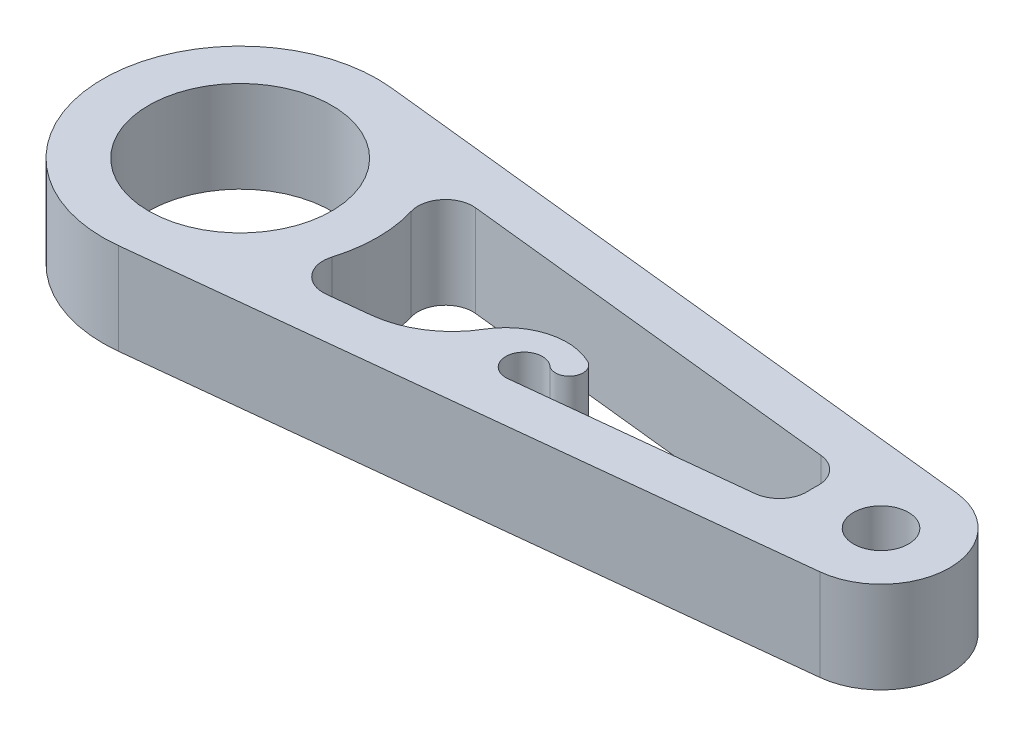
SolidWorks part; units mm, degrees
material "哈碳纤"
ref_plane "前视基准面" through (0, 0, 0) normal (0, 0, 1) x (1, 0, 0)
ref_plane "上视基准面" through (0, 0, 0) normal (0, 1, 0) x (1, 0, 0)
ref_plane "右视基准面" through (0, 0, 0) normal (1, 0, 0) x (0, 0, -1)
other "Configuration Table"
sketch "草图1" plane through (0, 0, 0) normal (0, 1, 0) x (1, 0, 0)
  line L0 (1.6071, 14.9137) -> (70.8036, 7.4568)
  line L1 (1.6071, -14.9137) -> (70.8036, -7.4568)
  line L2 (12.1874, 8.7445) -> (63.2375, 3.2432)
  line L3 (1.0714, 9.9424) -> (70.2679, 2.4856) construction
  line L4 (1.0714, -9.9424) -> (70.2679, -2.4856) construction
  line L5 (12.1874, -8.7445) -> (63.2375, -3.2432)
  circle A0 centre (0, 0) radius 10
  arc A1 (1.6071, 14.9137) -> (1.6071, -14.9137) centre (0, 0) ccw
  circle A2 centre (70, 0) radius 3
  arc A3 (70.8036, -7.4568) -> (70.8036, 7.4568) centre (70, 0) ccw
  arc A4 (12.1874, -8.7445) -> (12.1874, 8.7445) centre (0, 0) ccw
  arc A5 (63.2375, 3.2432) -> (63.2375, -3.2432) centre (70, 0) ccw
  dimension "D1" = 20
  dimension "D2" = 30
  dimension "D3" = 6
  dimension "D4" = 15
  dimension "D5" = 70
  dimension "D6" = 5
  dimension "D7" = 5
extrude "凸台-拉伸1" add sketch "草图1" along normal blind 10
fillet "圆角1" radius 3 4 edges at (63.2375, 5, 3.2432) (63.2375, 5, -3.2432) (12.1874, 5, 8.7445) (12.1874, 5, -8.7445)
sketch "草图2" plane through (0, 10, 0) normal (0, 1, 0) x (1, 0, 0)
  line L0 (-7.3229, 13.091) -> (-14.6458, 26.1821)
  line L2 (-14.6458, 26.1821) -> (-9.4094, 29.1112)
  line L3 (-9.4094, 29.1112) -> (1.6071, 14.9137)
  arc A0 (1.6071, 14.9137) -> (1.6071, -14.9137) centre (0, 0) ccw construction
  arc A1 (1.6071, 14.9137) -> (-7.3229, 13.091) centre (0, 0) ccw
  dimension "D2" = 30
  dimension "D3" = 6
extrude "凸台-拉伸2" [suppressed] add sketch "草图2" against normal blind 10
fillet "圆角2" [suppressed] radius 3
sketch "草图3" plane through (0, 10, 0) normal (0, 1, 0) x (1, 0, 0)
  line L0 (17.5591, -8.1657) -> (59.8401, -3.6093) construction
  line L1 (28.6131, -6.9745) -> (35.4729, -6.2352)
  arc A0 (36.559, -2.7272) -> (35.4729, -6.2352) centre (35.2586, -4.2467) ccw
  arc A1 (36.559, -2.7272) -> (38.1927, -0.2398) centre (37.5343, -1.5876) ccw
  arc A2 (38.1927, -0.2398) -> (28.6131, -6.9745) centre (35.2586, -6.2467) ccw
  circle A3 centre (70, 0) radius 3 construction
  point P1 (0, 0)
  point P3 (0, 0)
  point P13 (0, 0)
  point P14 (36.0991, -2.4319)
  point P15 (36.0955, -4.2741)
  dimension "D1" = 4
  dimension "D2" = 3
  dimension "D3" = 35
  dimension "D4" = 4.4
extrude "凸台-拉伸3" add sketch "草图3" against normal blind 10
fillet "圆角3" radius 10 1 edges at (28.6131, 5, 6.9745)
